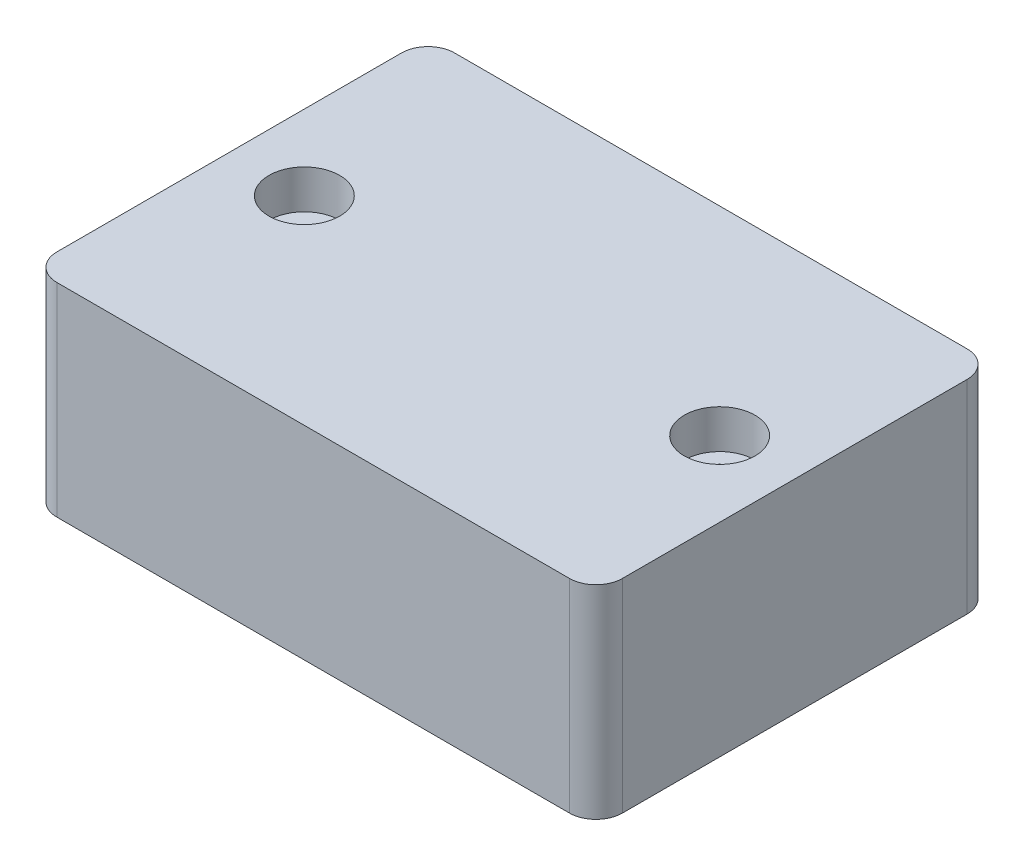
from build123d import *

# Parameters (mm, degrees)
SKETCH_1_W                   = 64
SKETCH_1_H                   = 45
EXTRUDE_1_DEPTH              = 11.5
HOLE_WIZARD_M4_1_D           = 4.5
HOLE_WIZARD_M4_1_CBORE_D     = 8
HOLE_WIZARD_M4_1_CBORE_DEPTH = 4.4
FILLET_1_R                   = 3


with BuildPart() as part:
    # 草图1 → 凸台-拉伸1 (new, symmetric)
    with BuildSketch(Plane(origin=(0, 0, 0), x_dir=(1, 0, 0), z_dir=(0, 1, 0))):
        Rectangle(SKETCH_1_W, SKETCH_1_H)
    extrude(amount=EXTRUDE_1_DEPTH, both=True)

    # M4 六角凹头螺钉的柱形沉头孔1 (through all)
    with Locations(Plane(origin=(0, 11.5, 0), x_dir=(1, 0, 0), z_dir=(0, 1, 0))):
        with Locations((-23.5, 0), (23.5, 0)):
            CounterBoreHole(HOLE_WIZARD_M4_1_D / 2, HOLE_WIZARD_M4_1_CBORE_D / 2, HOLE_WIZARD_M4_1_CBORE_DEPTH)

    # 圆角1
    fillet_1_edges = [part.edges().sort_by_distance(p)[0] for p in [
        (32, 0, 22.5),
        (-32, 0, 22.5),
        (-32, 0, -22.5),
        (32, 0, -22.5),
    ]]
    fillet(fillet_1_edges, radius=FILLET_1_R)


solid = part.part
